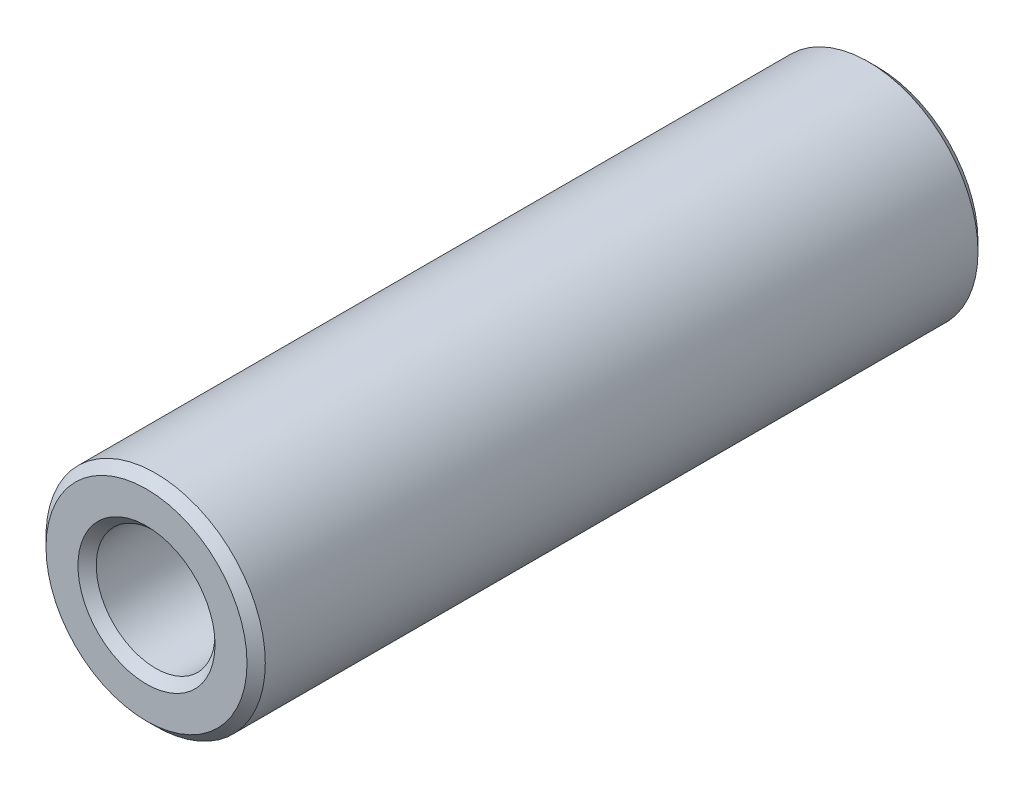
from build123d import *


with BuildPart() as part:
    # Sketch2 → Revolve1 (revolve)
    with BuildSketch(Plane(origin=(0, 0, 0), x_dir=(1, 0, 0), z_dir=(0, 1, 0))):
        Polygon((1.5, 0), (2.2, 0), (2.4, 0.2), (2.4, 15.8), (2.2, 16), (1.5, 16), (1.3, 15.8), (1.3, 0.2), align=None)
    revolve(axis=Axis((0, 0, 0), (0, 0, -1)))


solid = part.part
